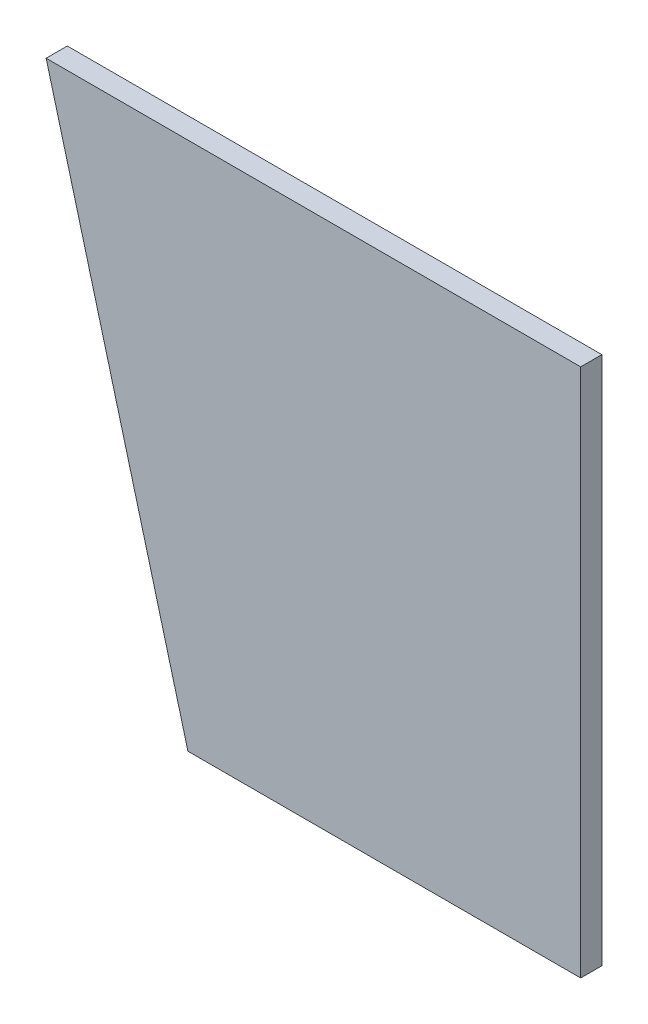
SolidWorks part; units mm, degrees
material "普通碳钢"
ref_plane "Front Plane" through (0, 0, 0) normal (0, 0, 1) x (1, 0, 0)
ref_plane "Top Plane" through (0, 0, 0) normal (0, 1, 0) x (1, 0, 0)
ref_plane "Right Plane" through (0, 0, 0) normal (1, 0, 0) x (0, 0, -1)
sketch "Sketch1" plane through (0, 0, 0) normal (0, 0, 1) x (1, 0, 0)
  line L0 (-303, 0) -> (0, 0)
  line L1 (0, 0) -> (0, -300)
  line L2 (0, -300) -> (-222.6152, -300)
  line L3 (-303, 0) -> (-222.6152, -300)
  dimension "D1" = 303
  dimension "D2" = 300
  dimension "D3" = 75
extrude "Extrude1" add sketch "Sketch1" along normal mid plane 12
